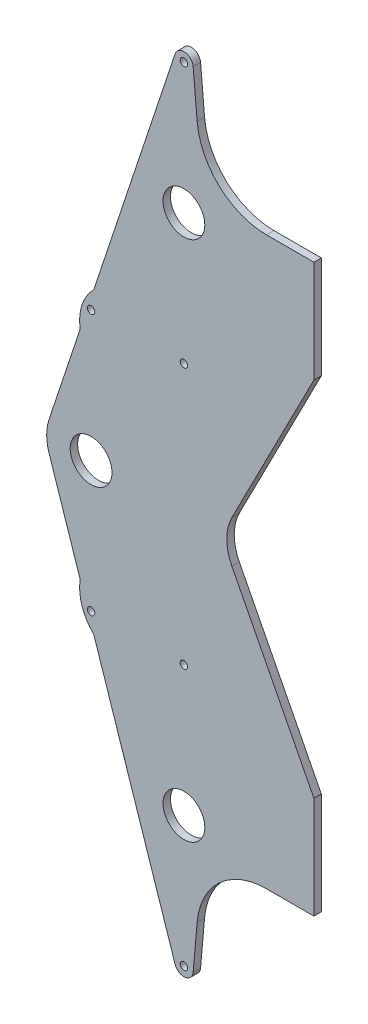
SolidWorks part; units mm, degrees
material "Q235B"
ref_plane "Front Plane" through (0, 0, 0) normal (0, 0, 1) x (1, 0, 0)
ref_plane "Top Plane" through (0, 0, 0) normal (0, 1, 0) x (1, 0, 0)
ref_plane "Right Plane" through (0, 0, 0) normal (1, 0, 0) x (0, 0, -1)
other "Configuration Table"
sketch "Sketch1" plane through (0, 0, 0) normal (0, 0, 1) x (1, 0, 0)
  line L0 (-102.0891, 610) -> (0, 610)
  line L1 (0, 610) -> (0, 390)
  line L2 (0, 390) -> (-176.5991, 45.6317)
  line L3 (-176.5991, -45.6317) -> (0, -390)
  line L4 (0, -390) -> (0, -610)
  line L5 (0, -610) -> (-233.9511, -610) construction
  line L6 (-570.5355, 31.514) -> (-503.4045, 233.6796)
  line L7 (-260.0761, 844.7431) -> (-251.5183, 746.9266)
  line L8 (-200, 0) -> (77.1778, 0) construction
  line L9 (-102.0891, -610) -> (0, -610)
  line L10 (-260.0761, -844.7431) -> (-251.5183, -746.9266)
  line L11 (-570.5355, -31.514) -> (-503.4045, -233.6796)
  line L12 (-480, -281) -> (-280, -281) construction
  line L13 (-480, -281) -> (-499.5661, -281) construction
  line L14 (-474.3367, -321.2173) -> (-298.9809, -849.3028)
  line L15 (-480, 281) -> (-499.5661, 281) construction
  line L16 (-480, 281) -> (-280, 281) construction
  line L17 (-487.9592, 280.1931) -> (-487.6913, 281)
  line L18 (-474.3367, 321.2173) -> (-298.9809, 849.3028)
  arc A1 (-260.0761, 844.7431) -> (-298.9809, 849.3028) centre (-280, 843) ccw
  arc A2 (-102.0891, 610) -> (-251.5183, 746.9266) centre (-102.0891, 760) cw
  arc A3 (-102.0891, -610) -> (-251.5183, -746.9266) centre (-102.0891, -760) ccw
  arc A4 (-260.0761, -844.7431) -> (-298.9809, -849.3028) centre (-280, -843) cw
  circle A5 centre (-480, 0) radius 45
  circle A6 centre (-280, -562) radius 45
  arc A7 (-503.4045, -233.6796) -> (-474.3367, -321.2173) centre (-404.6616, -249.486) ccw
  circle A8 centre (-480, -281) radius 8
  circle A9 centre (-280, -281) radius 8
  circle A10 centre (-280, -843) radius 8
  circle A11 centre (-280, 843) radius 8
  circle A12 centre (-405, 20) radius 3.5
  circle A13 centre (-405, -20) radius 3.5
  circle A14 centre (-355, -542) radius 3.5
  circle A15 centre (-355, -582) radius 3.5
  circle A16 centre (-280, 281) radius 8
  circle A17 centre (-480, 281) radius 8
  arc A18 (-503.4045, 233.6796) -> (-474.3367, 321.2173) centre (-404.6616, 249.486) cw
  circle A19 centre (-355, 582) radius 3.5
  circle A20 centre (-355, 542) radius 3.5
  circle A21 centre (-280, 562) radius 45
  arc A22 (-176.5991, 45.6317) -> (-176.5991, -45.6317) centre (-87.6174, 0) ccw
  arc A23 (-570.5355, 31.514) -> (-570.5355, -31.514) centre (-475.631, 0) ccw
  point P64 (-581, 0)
  dimension "D2" = 0
  dimension "D12" = 150
  dimension "D14" = 40
  dimension "D16" = 90
  dimension "D19" = 0
  dimension "D23" = 16
  dimension "D28" = 7
  dimension "D33" = 100
  dimension "D1" = 1220
  dimension "D3" = 220
  dimension "D4" = 220
  dimension "D5" = 0
  dimension "D6" = 200
  dimension "D7" = 0
  dimension "D8" = 843
  dimension "D9" = 581
  dimension "D10" = 0
  dimension "D11" = 280
  dimension "D13" = 610
  dimension "D15" = 95
  dimension "D17" = 480
  dimension "D18" = 562
  dimension "D20" = 200
  dimension "D21" = 0
  dimension "D22" = 281
  dimension "D24" = 40
  dimension "D25" = 20
  dimension "D26" = 75
  dimension "D27" = 75
  dimension "D29" = 20
  dimension "D30" = 20
  dimension "D31" = 75
  dimension "D32" = 75
extrude "Boss-Extrude1" add sketch "Sketch1" along normal blind 16 contours L6 A23 L11 A7 L14 A4 L10 A3 L9 L4 L3 A22 L2 L1 L0 A2 L7 A1 L18 A18 A21 A19 A16 A15 A14 A13 A12 A11 A10 A9 A8 A6 A5 A17 A20
hole_wizard "M10 Tapped Hole1" positions "Sketch2" profile "Sketch3" tap size "M10" standard "GB"
sketch "Sketch2" plane through (0, 0, 16) normal (0, 0, 1) x (1, 0, 0)
  point P0 (-405, -20)
  point P3 (-405, 20)
  point P6 (-355, -542)
  point P9 (-355, -582)
  point P12 (-355, 582)
  point P15 (-355, 542)
sketch "Sketch3" plane through (-405, -20, 16) normal (1, 0, 0) x (0, -1, 0)
  line L0 (0, 0) -> (0, 16)
  line L1 (0, 16) -> (4.25, 16)
  line L2 (4.25, 16) -> (4.25, 0)
  line L5 (4.25, 0) -> (0, 0)
  line L11 (0, -6.35) -> (0, 107.95) construction
  dimension "通孔螺纹孔钻头直径" = 8.5
  dimension "通孔螺纹孔钻头深度" = 16
cosmetic thread "Hole Thread1" [suppressed] parameters "D2"=10
cosmetic thread "Hole Thread2" [suppressed] parameters "D2"=10
cosmetic thread "Hole Thread3" [suppressed] parameters "D2"=10
cosmetic thread "Hole Thread4" [suppressed] parameters "D2"=10
cosmetic thread "Hole Thread5" [suppressed] parameters "D2"=10
cosmetic thread "Hole Thread6" [suppressed] parameters "D2"=10
sketch "Sketch4" plane through (0, 0, 16) normal (0, 0, 1) x (1, 0, 0)
  circle A0 centre (-355, -542) radius 3.5 construction
  circle A1 centre (-355, -582) radius 3.5 construction
  circle A2 centre (-405, -20) radius 3.5 construction
  circle A3 centre (-405, 20) radius 3.5 construction
  circle A4 centre (-355, 542) radius 3.5 construction
  circle A5 centre (-355, 582) radius 3.5 construction
  circle A6 centre (-355, -542) radius 3.5
  circle A7 centre (-355, -582) radius 3.5
  circle A8 centre (-405, -20) radius 3.5
  circle A9 centre (-405, 20) radius 3.5
  circle A10 centre (-355, 542) radius 3.5
  circle A11 centre (-355, 582) radius 3.5
extrude "Boss-Extrude2" add sketch "Sketch4" against normal up to surface (16 mm away) up to face at (-235, 562, 0)
equation "\"281cm.\"=270.41"
